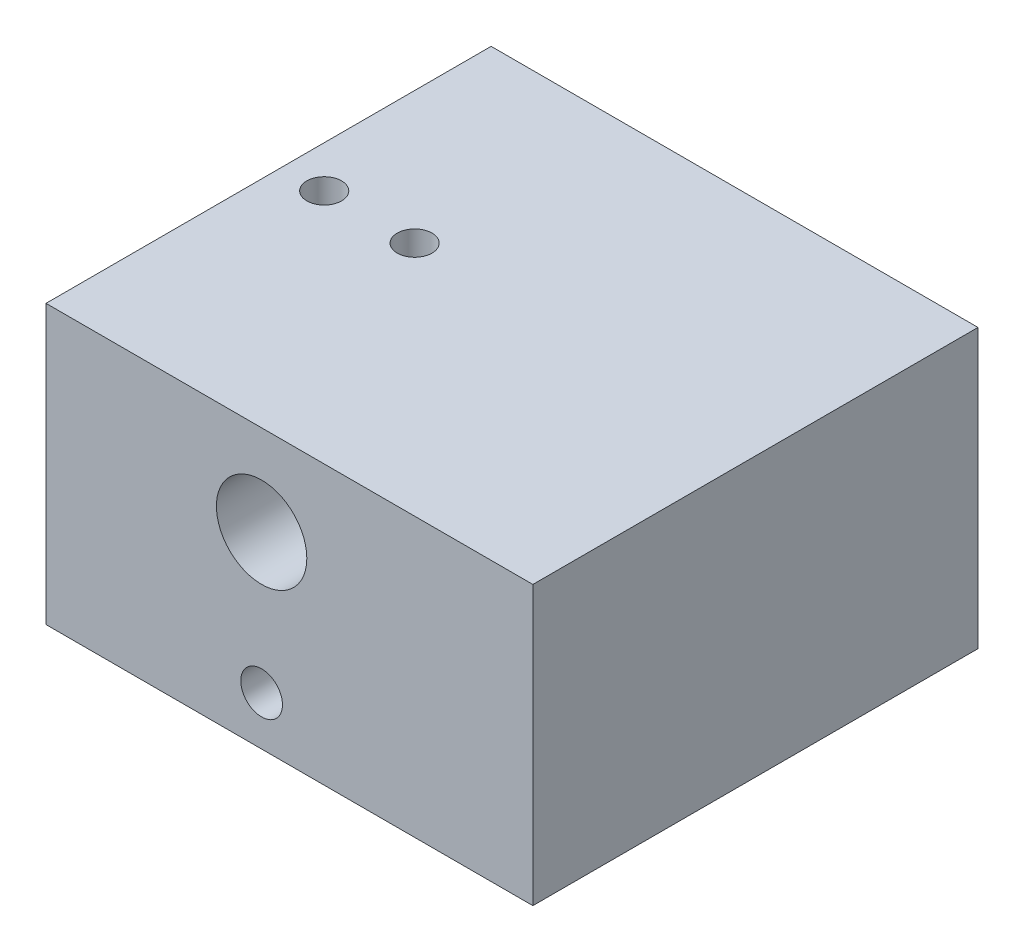
SolidWorks part; units mm, degrees
material "20#"
ref_plane "Front Plane" through (0, 0, 0) normal (0, 0, 1) x (1, 0, 0)
ref_plane "Top Plane" through (0, 0, 0) normal (0, 1, 0) x (1, 0, 0)
ref_plane "Right Plane" through (0, 0, 0) normal (1, 0, 0) x (0, 0, -1)
sketch "Sketch1" plane through (0, 0, 0) normal (0, 1, 0) x (1, 0, 0)
  line L1 (-17.5, 16) -> (17.5, 16)
  line L2 (-17.5, 16) -> (-17.5, -16)
  line L3 (-17.5, -16) -> (17.5, -16)
  line L4 (17.5, 16) -> (17.5, -16)
  line L5 (-17.5, 16) -> (17.5, -16) construction
  line L6 (-17.5, -16) -> (17.5, 16) construction
  point P0 (0, 0)
  dimension "D1" = 35
  dimension "D2" = 32
extrude "Boss-Extrude1" add sketch "Sketch1" along normal blind 20
sketch "Sketch3" plane through (0, 0, 16) normal (0, 0, 1) x (1, 0, 0)
  line L0 (17.5, 20) -> (-17.5, 20) construction
  circle A0 centre (-2, 13.5) radius 3.25
  circle A1 centre (-2, 3.5) radius 1.5
  dimension "D1" = 6.5
  dimension "D2" = 3
  dimension "D3" = 10
  dimension "D4" = 6.5
  dimension "D5" = 2
extrude "Cut-Extrude2" cut sketch "Sketch3" against normal up to next
sketch "Sketch4" plane through (0, 20, 0) normal (0, 1, 0) x (1, 0, 0)
  circle A0 centre (-8, 1) radius 1
  circle A1 centre (-14.5, 1) radius 1
  dimension "D1" = 2
extrude "Cut-Extrude3" cut sketch "Sketch4" against normal blind 2
hole_wizard "M3 Tapped Hole1" positions "Sketch5" profile "Sketch6" tap size "M3" standard "GB"
sketch "Sketch5" plane through (0, 20, 0) normal (0, 1, 0) x (1, 0, 0)
  point P0 (-8, 1)
  point P3 (-14.5, 1)
sketch "Sketch6" plane through (-8, 20, -1) normal (1, 0, 0) x (0, 0, 1)
  line L0 (0, 0) -> (0, 8.2511)
  line L1 (0, 8.2511) -> (1.25, 7.5)
  line L2 (1.25, 7.5) -> (1.25, 0)
  line L5 (1.25, 0) -> (0, 0)
  line L10 (0, 8.2511) -> (-1.25, 7.5) construction
  line L11 (0, -6.35) -> (0, 107.95) construction
  dimension "螺纹孔钻头直径" = 2.5
  dimension "螺纹孔钻头深度" = 7.5
  dimension "导头角度" = 118
cosmetic thread "HoleThreadLine2" parameters "D1"=6, "D2"=3
cosmetic thread "HoleThreadLine3" parameters "D1"=6, "D2"=3
